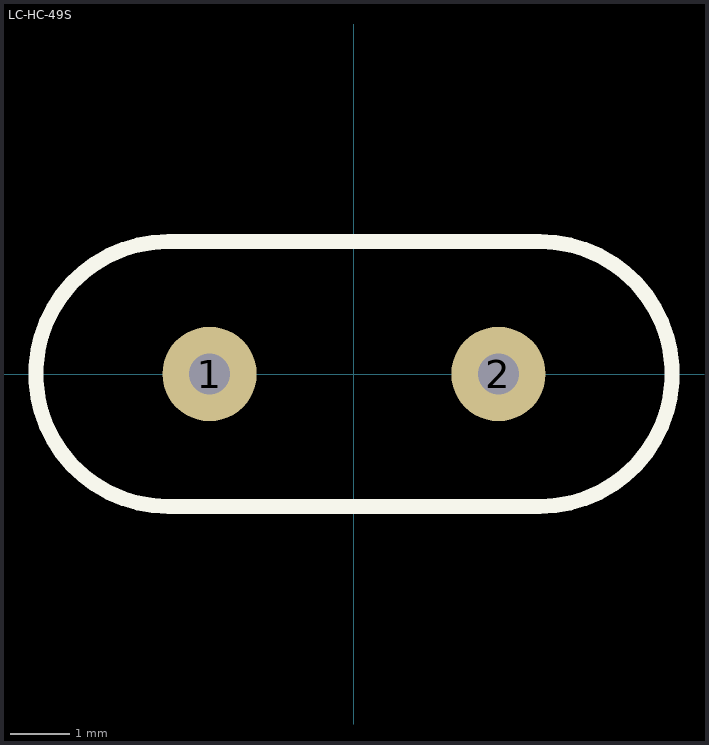
[diagram p0: the footprint, top view; thin cyan lines are the x and y axes]
# Altium footprint library MISC89340-23.PcbLib: 1 footprints
Each footprint in its own frame and in the unit in brackets; x right, y up, seen from the top. Pads: shape width x height; smd on the part's side, far side on the other; paste and mask are expansions set on the pad; w line width, h text height; cw(c..) or ccw(c..) is an arc to the next point about the centre after c.

## LC-HC-49S [mm]
pads (2):
  round 1.6 hole 0.7: 1(-2.45,0) 2(2.45,0)
Top Overlay:
  lines w0.254: -3.15,-2.248 cw(c-3.15,0) -3.15,2.248 3.15,2.248 cw(c3.15,0) 3.15,-2.248 -3.15,-2.248